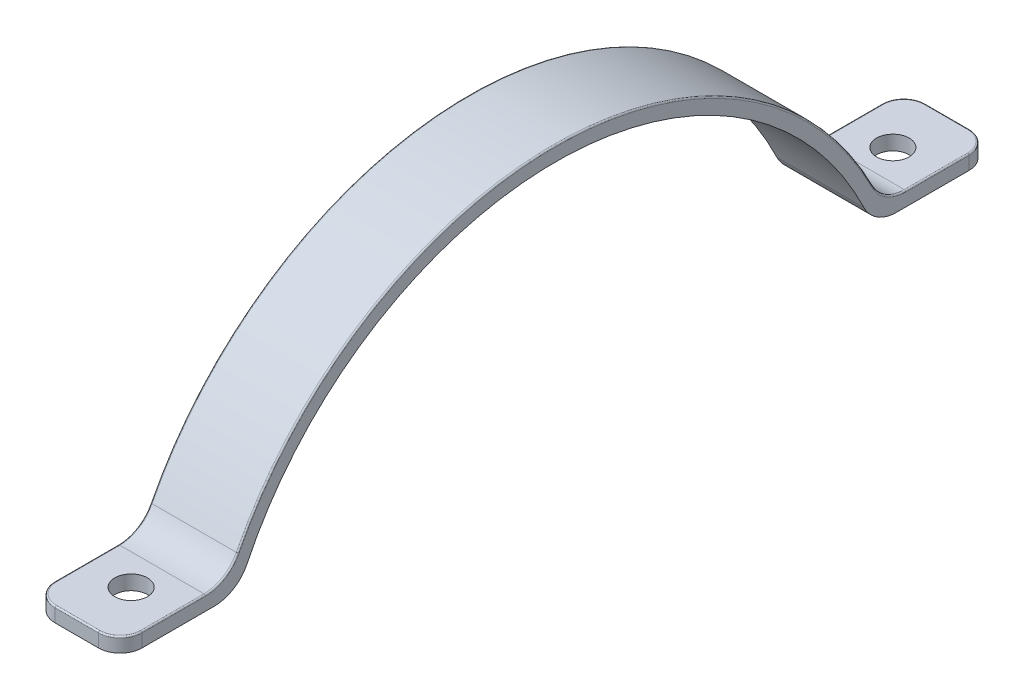
from build123d import *

# Parameters (mm, degrees)
EXTRUDE_1_DEPTH     = 6
SKETCH_2_R          = 2.25
CUT_EXTRUDE_1_DEPTH = 12
FILLET_1_R          = 3
FILLET_2_R          = 5
FILLET_3_R          = 5
FILLET_4_R          = 0.2


with BuildPart() as part:
    # 草图1 → 凸台-拉伸1 (new, symmetric)
    with BuildSketch(Plane(origin=(0, 0, 0), x_dir=(0, 0, -1), z_dir=(1, 0, 0))):
        with BuildLine():
            Line((43.757393596, 17.659225719), (60, 17.659225719))
            Line((60, 17.659225719), (60, 19.659225719))
            Line((60, 19.659225719), (45.097063909, 19.659225719))
            ThreePointArc((45.097063909, 19.659225719), (0, 49.195836501), (-45.097063909, 19.659225719))
            Line((-45.097063909, 19.659225719), (-60, 19.659225719))
            Line((-60, 19.659225719), (-60, 17.659225719))
            Line((-60, 17.659225719), (-43.757393596, 17.659225719))
            ThreePointArc((-43.757393596, 17.659225719), (0, 47.186414859), (43.757393596, 17.659225719))
        make_face()
    extrude(amount=EXTRUDE_1_DEPTH, both=True)

    # 草图2 → 切除-拉伸1 (cut)
    with BuildSketch(Plane(origin=(0, 19.659225719, 0), x_dir=(1, 0, 0), z_dir=(0, 1, 0))):
        with Locations(Location((0, -52.5, 0), (0, 0, 270))):
            Circle(SKETCH_2_R)
        with Locations(Location((0, 52.5, 0), (0, 0, 270))):
            Circle(SKETCH_2_R)
    extrude(amount=-CUT_EXTRUDE_1_DEPTH, mode=Mode.SUBTRACT)

    # 圆角1
    fillet_1_edges = [part.edges().sort_by_distance(p)[0] for p in [
        (6, 18.659225719, -60),
        (6, 18.659225719, 60),
        (-6, 18.659225719, 60),
        (-6, 18.659225719, -60),
    ]]
    fillet(fillet_1_edges, radius=FILLET_1_R)

    # 圆角2
    fillet_2_edges = [part.edges().sort_by_distance(p)[0] for p in [
        (0, 19.659225719, 45.097063909),
        (0, 19.659225719, -45.097063909),
    ]]
    fillet(fillet_2_edges, radius=FILLET_2_R)

    # 圆角3
    fillet_3_edges = [part.edges().sort_by_distance(p)[0] for p in [
        (0, 17.659225719, 43.757393596),
        (0, 17.659225719, -43.757393596),
    ]]
    fillet(fillet_3_edges, radius=FILLET_3_R)

    # 圆角4
    fillet_4_edges = [part.edges().sort_by_distance(p)[0] for p in [
        (6, 19.659225719, -52.630433487),
        (0, 19.659225719, 60),
        (-5.121320344, 19.659225719, 59.121320344),
        (5.121320344, 19.659225719, 59.121320344),
        (-6, 19.659225719, -52.630433487),
        (0, 19.659225719, -60),
        (5.121320344, 19.659225719, -59.121320344),
        (-5.121320344, 19.659225719, -59.121320344),
        (-6, 49.195836501, 0),
        (6, 49.195836501, 0),
        (6, 19.659225719, 52.630433487),
        (-6, 19.659225719, 52.630433487),
        (-6, 20.394541943, -45.650795653),
        (6, 20.394541943, -45.650795653),
        (-6, 20.394541943, 45.650795653),
        (6, 20.394541943, 45.650795653),
    ]]
    fillet(fillet_4_edges, radius=FILLET_4_R)


solid = part.part
